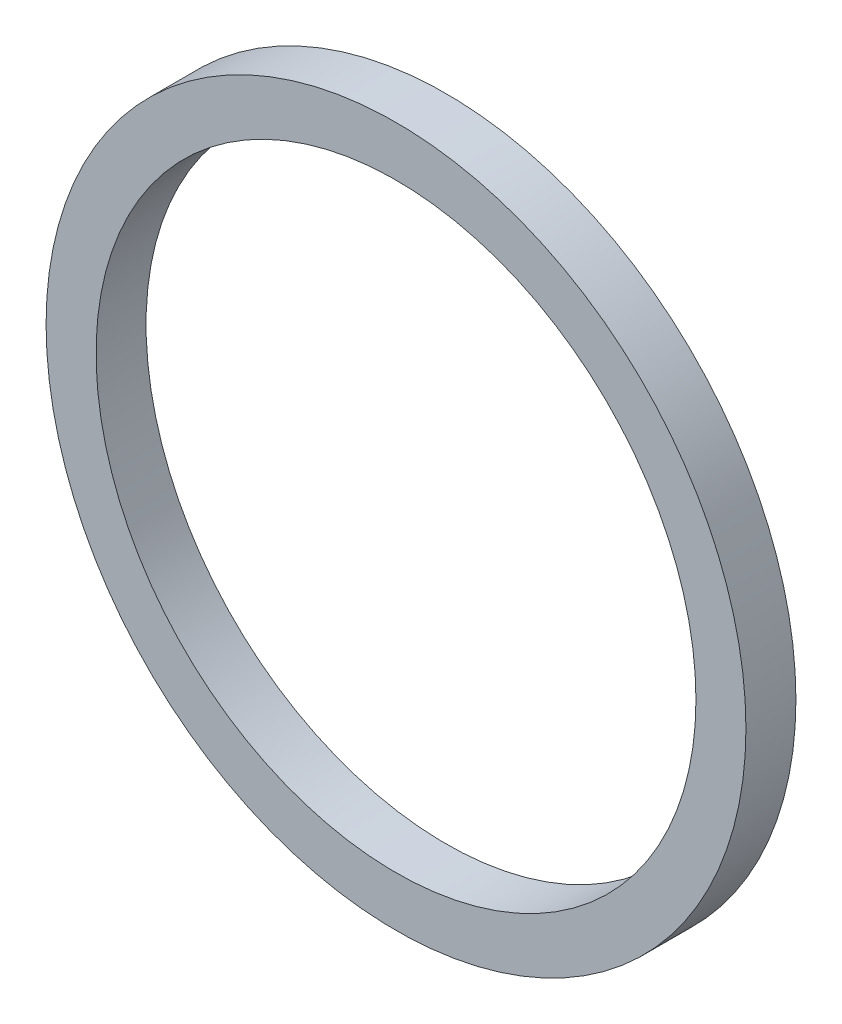
from build123d import *

# Parameters (mm, degrees)
SKETCH_1_R      = 17.5
SKETCH_1_R_2    = 15
EXTRUDE_1_DEPTH = 2.5


with BuildPart() as part:
    # 草图1 → 凸台-拉伸1 (new body)
    with BuildSketch(Plane.XY):
        Circle(SKETCH_1_R)
        Circle(SKETCH_1_R_2, mode=Mode.SUBTRACT)
    extrude(amount=EXTRUDE_1_DEPTH)


solid = part.part
